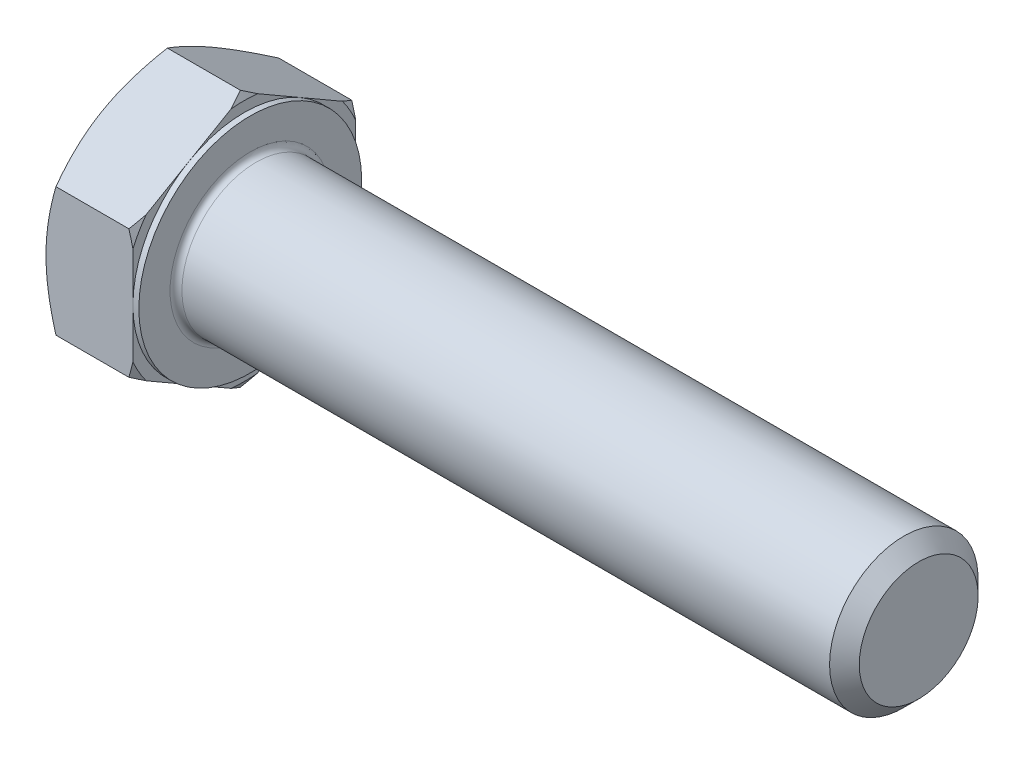
from build123d import *

# Parameters (mm, degrees)
EXTRUDE_365_DEPTH = 12.5
SKETCH_4_W        = 0.8
SKETCH_4_H        = 12.320508076
CHAMFER_2074_SIZE = 2
FILLET_2128_R     = 0.8


with BuildPart() as part:
    # 草图1 → Extrude 365 (new body)
    with BuildSketch(Plane(origin=(0, 0, 0), x_dir=(0, 0, -1), z_dir=(1, 0, 0))):
        Polygon((15, 8.660254038), (15, -8.660254038), (0, -17.320508076), (-15, -8.660254038), (-15, 8.660254038), (0, 17.320508076), align=None)
    extrude(amount=EXTRUDE_365_DEPTH)

    # 草图2 → 凸台-旋转1 (revolve)
    with BuildSketch(Plane.XY, mode=Mode.PRIVATE) as revolve_1_sk:
        Polygon((0, 0), (102.5, 0), (102.5, 7.835), (102.5, 10), (7.791693541, 10), (0, 10), align=None)
    revolve(revolve_1_sk.sketch.rotate(Axis((0, 0, 0), (1, 0, 0)), 90), axis=Axis((0, 0, 0), (1, 0, 0)))

    # 草图3 → 切除-旋转1 (revolve, cut)
    with BuildSketch(Plane.XY):
        Polygon((0, 15), (4.226497308, 22.320508076), (4.226497308, 27.320508076), (-10, 27.320508076), (-10, 15), align=None)
    revolve(axis=Axis((0, 0, 0), (1, 0, 0)), mode=Mode.SUBTRACT)

    # 草图5 → 切除-旋转2 (revolve, cut)
    with BuildSketch(Plane.XY):
        Polygon((12.5, 15), (8.273502692, 22.320508076), (8.273502692, 27.320508076), (18.273502692, 27.320508076), (18.273502692, 15), align=None)
    revolve(axis=Axis((0, 0, 0), (1, 0, 0)), mode=Mode.SUBTRACT)

    # 草图4 → 切除-旋转3 (revolve, cut)
    with BuildSketch(Plane.XY, mode=Mode.PRIVATE) as cut_revolve_3_sk:
        with Locations((12.1, 21.160254038)):
            Rectangle(SKETCH_4_W, SKETCH_4_H)
    revolve(cut_revolve_3_sk.sketch.rotate(Axis((0, 0, 0), (1, 0, 0)), 270), axis=Axis((0, 0, 0), (1, 0, 0)), mode=Mode.SUBTRACT)

    # Chamfer 2074
    chamfer_2074_edges = [part.edges().sort_by_distance(p)[0] for p in [
        (102.5, 0, -10),
    ]]
    chamfer(chamfer_2074_edges, length=CHAMFER_2074_SIZE)

    # Fillet 2128
    fillet_2128_edges = [part.edges().sort_by_distance(p)[0] for p in [
        (12.5, 0, -10),
    ]]
    fillet(fillet_2128_edges, radius=FILLET_2128_R)


solid = part.part
